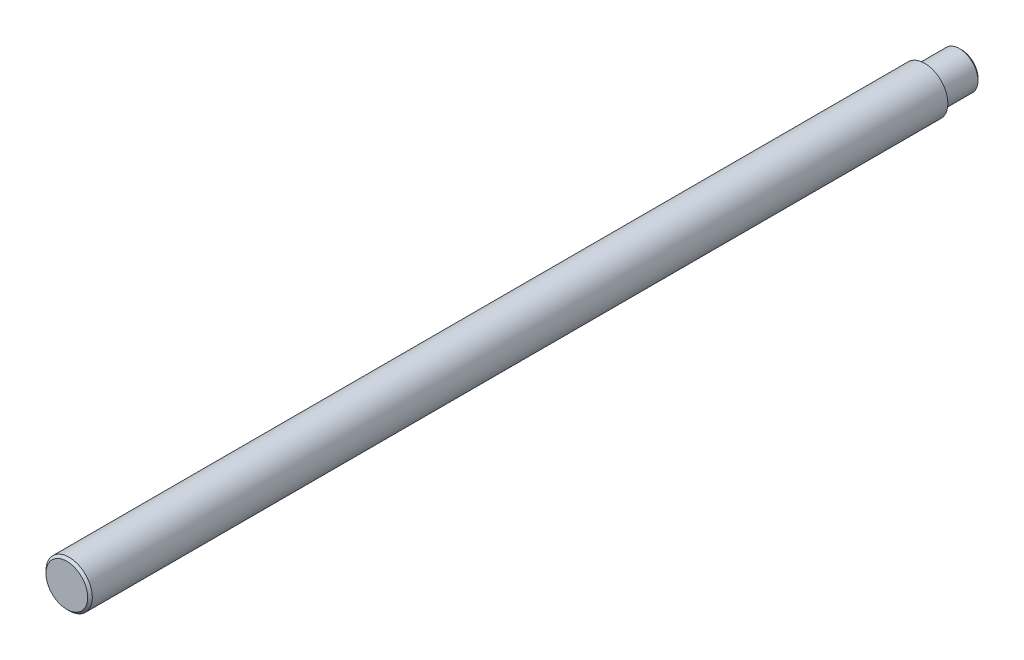
SolidWorks part; units mm, degrees
ref_plane "前视基准面" through (0, 0, 0) normal (0, 0, 1) x (1, 0, 0)
ref_plane "上视基准面" through (0, 0, 0) normal (0, 1, 0) x (1, 0, 0)
ref_plane "右视基准面" through (0, 0, 0) normal (1, 0, 0) x (0, 0, -1)
sketch "草图1" plane through (0, 0, 0) normal (0, 0, 1) x (1, 0, 0)
  circle A0 centre (0, 0) radius 5
  dimension "D1" = 10
extrude "凸台-拉伸1" add sketch "草图1" along normal blind 185
sketch "草图2" plane through (0, 0, 0) normal (0, 0, -1) x (-1, 0, 0)
  circle A0 centre (0, 0) radius 4
  dimension "D1" = 8
extrude "凸台-拉伸2" add sketch "草图2" along normal blind 8
chamfer "倒角1" distance 0.5 angle 45 2 edges at (-4, 0, -8) (5, 0, 185)
